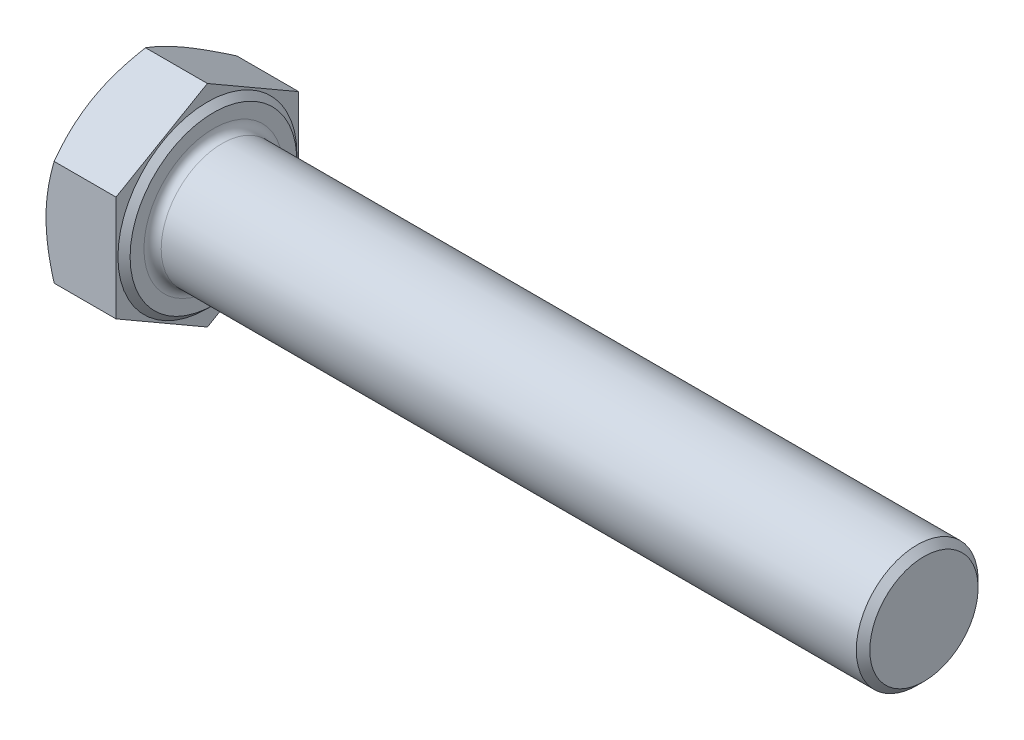
from build123d import *

# Parameters (mm, degrees)
BOSS_EXTRUDE1_DEPTH = 7.5
SKETCH4_R           = 20.03
SKETCH4_R_2         = 9
CUT_EXTRUDE1_DEPTH  = 0.9375
CUT_EXTRUDE1_DRAFT  = -60
CHAMFER2_SIZE       = 0.666666667


with BuildPart() as part:
    # Sketch3 → Boss-Extrude1 (new body)
    with BuildSketch(Plane(origin=(0, 0, 0), x_dir=(0, 0, -1), z_dir=(1, 0, 0))):
        Polygon((9, 5.196152423), (0, 10.392304845), (-9, 5.196152423), (-9, -5.196152423), (0, -10.392304845), (9, -5.196152423), align=None)
    extrude(amount=BOSS_EXTRUDE1_DEPTH)


with BuildPart() as cut_extrude1_tool:
    # Sketch4 → Cut-Extrude1 (with draft: the straight prism first)
    with BuildSketch(Plane.ZY):
        Circle(SKETCH4_R)
        Circle(SKETCH4_R_2, mode=Mode.SUBTRACT)
    extrude(amount=-CUT_EXTRUDE1_DEPTH)
    # Cut-Extrude1: the draft: its side faces are tilted about the plane it starts from
    cut_extrude1_sides = [cut_extrude1_tool.faces().sort_by_distance(p)[0] for p in [
        (0.46875, 0, -20.03),
        (0.46875, 0, -9),
    ]]
    draft(cut_extrude1_sides, Plane.ZY, CUT_EXTRUDE1_DRAFT)


with BuildPart() as part_1:
    add(part.part)

    # Cut-Extrude1: cut by cut_extrude1_tool
    add(cut_extrude1_tool.part, mode=Mode.SUBTRACT)

    # Sketch5 → Revolve1 (revolve)
    with BuildSketch(Plane.XY, mode=Mode.PRIVATE) as revolve1_sk:
        with BuildLine():
            Line((8.35, 6), (77.5, 6))
            Line((77.5, 6), (77.5, 0))
            Line((77.5, 0), (7.5, 0))
            Line((7.5, 0), (7.5, 6.85))
            ThreePointArc((7.5, 6.85), (7.748959236, 6.248959236), (8.35, 6))
        make_face()
    revolve(revolve1_sk.sketch.rotate(Axis((7.5, 0, 0), (1, 0, 0)), 90), axis=Axis((7.5, 0, 0), (1, 0, 0)))

    # Chamfer2
    chamfer2_edges = [part_1.edges().sort_by_distance(p)[0] for p in [
        (77.5, 0, -6),
    ]]
    chamfer(chamfer2_edges, length=CHAMFER2_SIZE)

    # Sketch7 → Cut-Revolve1 (revolve, cut)
    with BuildSketch(Plane.XY, mode=Mode.PRIVATE) as cut_revolve1_sk:
        Polygon((7.5, 8.215), (6.9, 8.815), (6.9, 20.03), (7.5, 20.03), align=None)
    revolve(cut_revolve1_sk.sketch.rotate(Axis((0, 0, 0), (1, 0, 0)), 90), axis=Axis((0, 0, 0), (1, 0, 0)), mode=Mode.SUBTRACT)


solid = part_1.part
